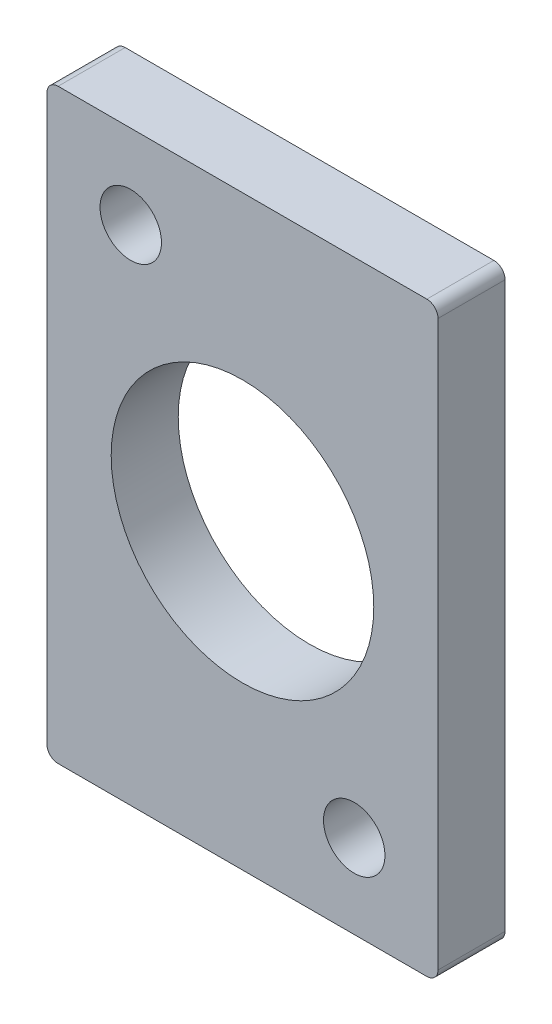
SolidWorks part; units mm, degrees
ref_plane "前视基准面" through (0, 0, 0) normal (0, 0, 1) x (1, 0, 0)
ref_plane "上视基准面" through (0, 0, 0) normal (0, 1, 0) x (1, 0, 0)
ref_plane "右视基准面" through (0, 0, 0) normal (1, 0, 0) x (0, 0, -1)
sketch "草图1" plane through (0, 0, 0) normal (0, 0, 1) x (1, 0, 0)
  line L1 (-33, 52.5) -> (33, 52.5)
  line L2 (-35, 50.5) -> (-35, -50.5)
  line L3 (-33, -52.5) -> (33, -52.5)
  line L4 (35, 50.5) -> (35, -50.5)
  line L5 (-35, 52.5) -> (35, -52.5) construction
  line L6 (-35, -52.5) -> (35, 52.5) construction
  circle A1 centre (0, 0) radius 23.5
  circle A2 centre (-20, 37.5) radius 5.5
  circle A3 centre (20, -37.5) radius 5.5
  arc A4 (-33, 52.5) -> (-35, 50.5) centre (-33, 50.5) ccw
  arc A5 (33, 52.5) -> (35, 50.5) centre (33, 50.5) cw
  arc A6 (33, -52.5) -> (35, -50.5) centre (33, -50.5) ccw
  arc A7 (-35, -50.5) -> (-33, -52.5) centre (-33, -50.5) ccw
  point P0 (0, 0)
  dimension "D3" = 47
  dimension "D4" = 11
  dimension "D9" = 2
  dimension "D1" = 70
  dimension "D2" = 105
  dimension "D5" = 15
  dimension "D6" = 15
  dimension "D7" = 15
  dimension "D8" = 15
extrude "凸台-拉伸1" add sketch "草图1" along normal blind 12
